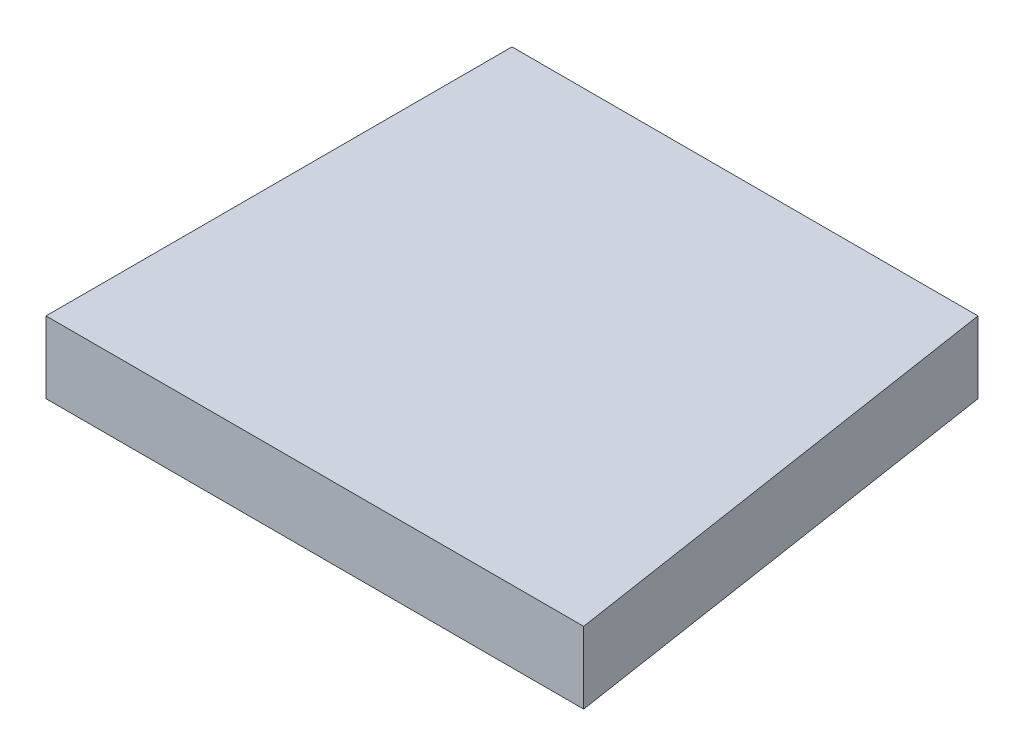
from build123d import *

# Parameters (mm, degrees)
EXTRUDE_1_DEPTH = 4


with BuildPart() as part:
    # 草图1 → 凸台-拉伸1 (new body)
    with BuildSketch(Plane(origin=(0, 0, 0), x_dir=(1, 0, 0), z_dir=(0, 1, 0))):
        Polygon((0, 0), (0, 26), (26, 26), (30, 0), align=None)
    extrude(amount=EXTRUDE_1_DEPTH)


solid = part.part
